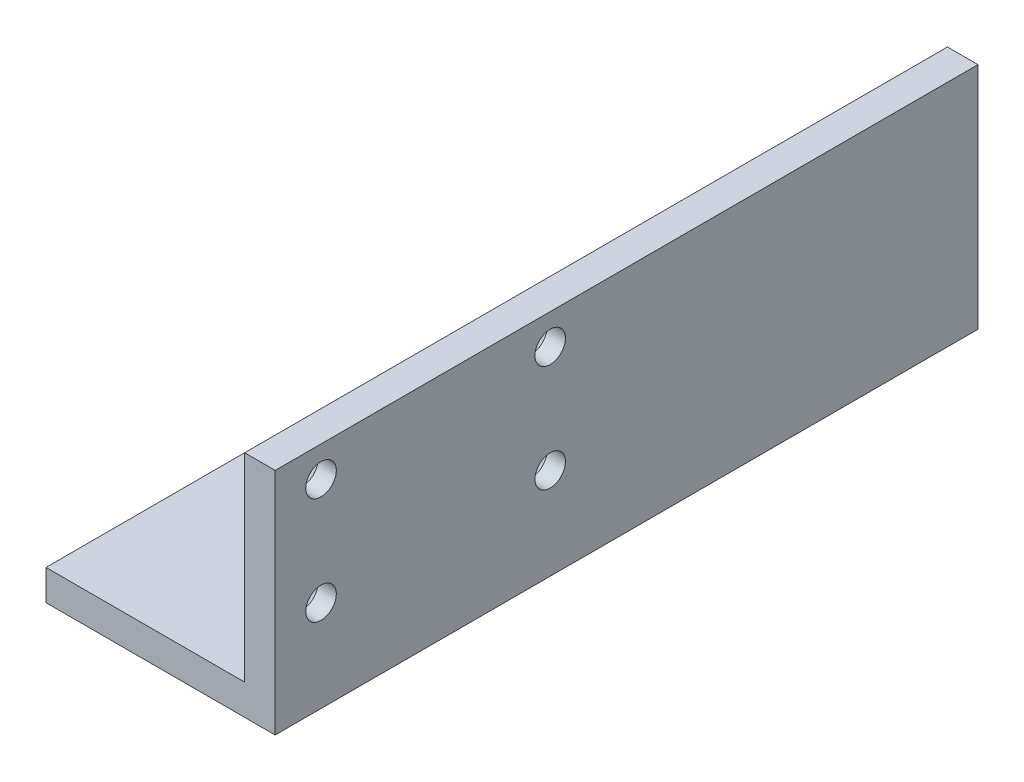
from build123d import *

# Parameters (mm, degrees)
EXTRUDE_1_DEPTH              = 50
HOLE_WIZARD_M8_1_D           = 10
HOLE_WIZARD_M8_1_CSINK_D     = 17.92
HOLE_WIZARD_M8_1_CSINK_ANGLE = 90
MOVE_FACE_1_BY               = 130
HOLE_WIZARD_M8_1_2_D         = 10


with BuildPart() as part:
    # 草图1 → 凸台-拉伸1 (new, symmetric)
    with BuildSketch(Plane.XY):
        Polygon((0, 0), (75, 0), (75, 75), (65, 75), (65, 10), (0, 10), align=None)
    extrude(amount=EXTRUDE_1_DEPTH, both=True)

    # Hole Wizard M8 _1 (through all)
    with Locations(Plane.ZY.offset(-65)):
        with Locations((-40, 65), (35, 65), (-40, 30), (35, 30)):
            CounterSinkHole(HOLE_WIZARD_M8_1_D / 2, HOLE_WIZARD_M8_1_CSINK_D / 2, counter_sink_angle=HOLE_WIZARD_M8_1_CSINK_ANGLE)

    # Move Face 1: a face moved outward by 130.0
    extrude(part.faces().sort_by_distance((37.5, 7.5, -50))[0], amount=MOVE_FACE_1_BY, dir=(0, 0, -1))

    # Hole Wizard M8 _1 2 (through all)
    with Locations(Plane(origin=(0, 10, 0), x_dir=(1, 0, 0), z_dir=(0, 1, 0))):
        with Locations((10.5, 165), (10.5, 95), (44.5, 165), (44.5, 95)):
            Hole(HOLE_WIZARD_M8_1_2_D / 2)


solid = part.part
